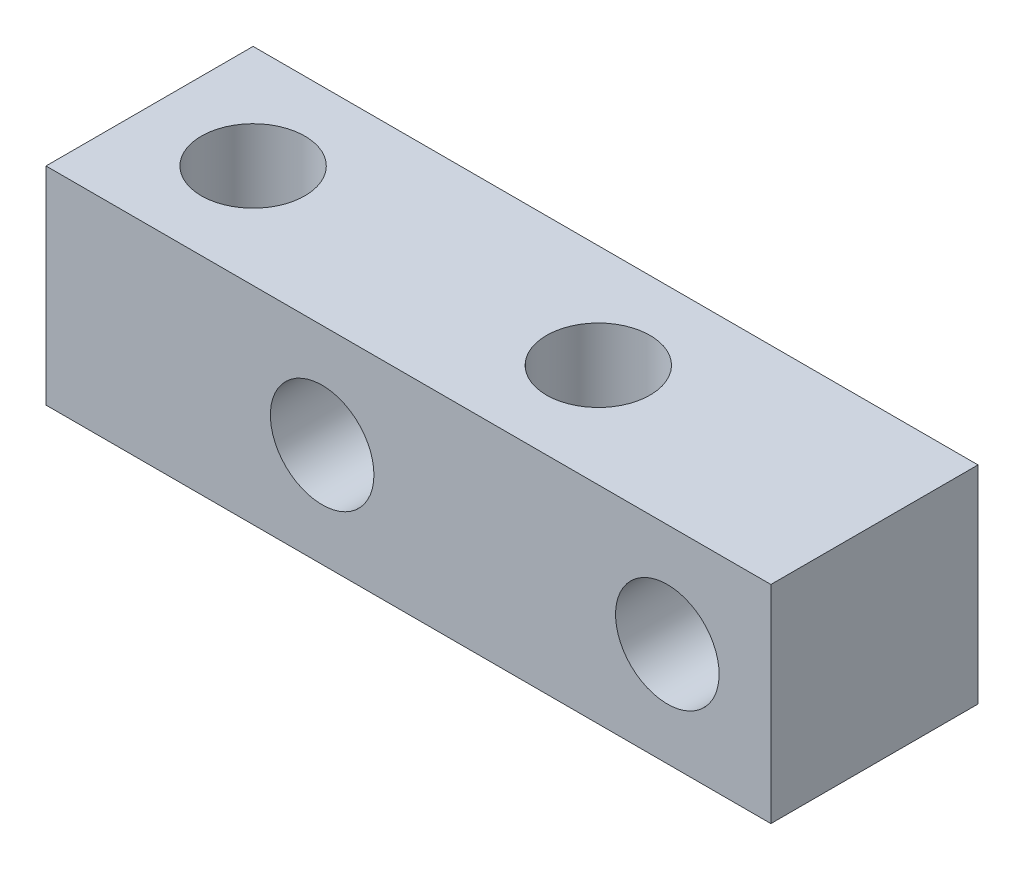
from build123d import *

# Parameters (mm, degrees)
SKETCH_1_W          = 21
SKETCH_1_H          = 6
SKETCH_1_R          = 1.5
EXTRUDE_1_DEPTH     = 6
SKETCH_2_R          = 1.5
CUT_EXTRUDE_1_DEPTH = 23.649503306


with BuildPart() as part:
    # 草图1 → 凸台-拉伸1 (new body)
    with BuildSketch(Plane(origin=(0, 0, 0), x_dir=(1, 0, 0), z_dir=(0, 1, 0))):
        with Locations((10.5, 3)):
            Rectangle(SKETCH_1_W, SKETCH_1_H)
        with Locations(Location((3, 3, 0), (0, 0, 270))):
            Circle(SKETCH_1_R, mode=Mode.SUBTRACT)
        with Locations(Location((13, 3, 0), (0, 0, 270))):
            Circle(SKETCH_1_R, mode=Mode.SUBTRACT)
    extrude(amount=EXTRUDE_1_DEPTH)

    # 草图2 → 切除-拉伸1 (cut, through all)
    with BuildSketch(Plane.XY):
        with Locations((18, 3)):
            Circle(SKETCH_2_R)
        with Locations((8, 3)):
            Circle(SKETCH_2_R)
    extrude(amount=-CUT_EXTRUDE_1_DEPTH, mode=Mode.SUBTRACT)


solid = part.part
